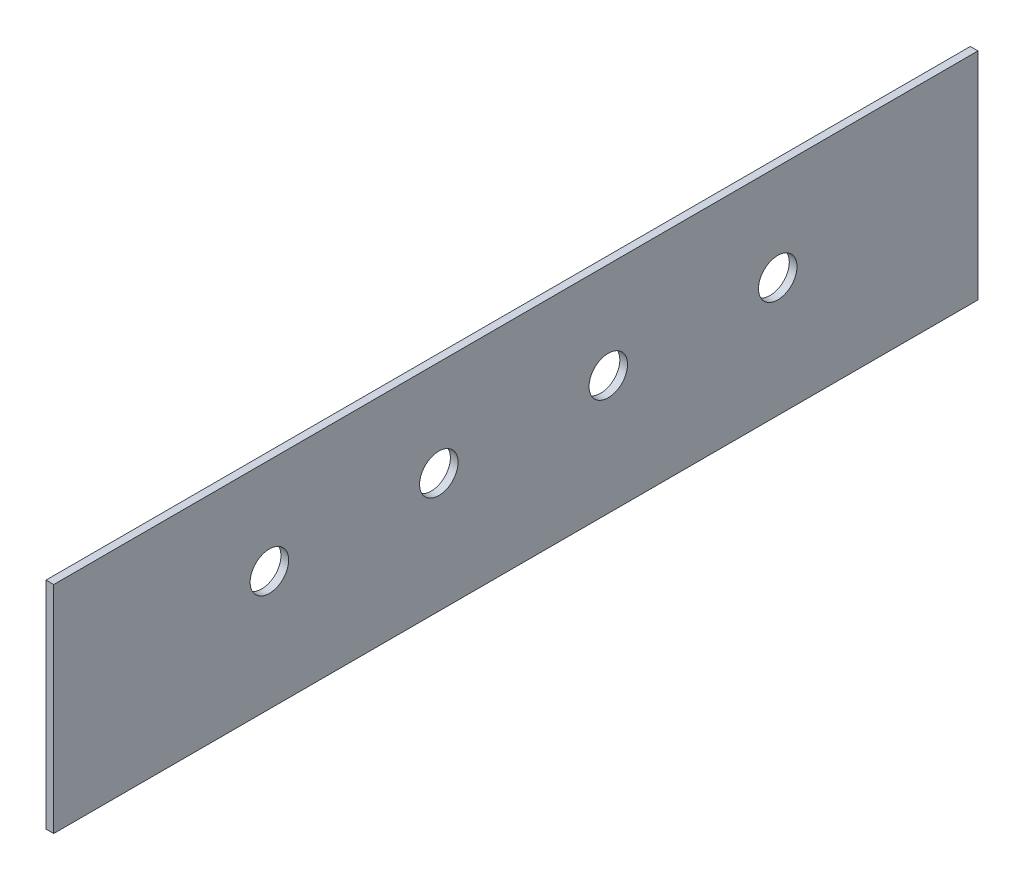
SolidWorks part; units mm, degrees
ref_plane "Front Plane" through (0, 0, 0) normal (0, 0, 1) x (1, 0, 0)
ref_plane "Top Plane" through (0, 0, 0) normal (0, 1, 0) x (1, 0, 0)
ref_plane "Right Plane" through (0, 0, 0) normal (1, 0, 0) x (0, 0, -1)
other "Configuration Table"
sketch "Sketch1" plane through (0, 0, 0) normal (1, 0, 0) x (0, 0, -1)
  line L1 (-600, -140) -> (600, -140)
  line L2 (-600, -140) -> (-600, 140)
  line L3 (-600, 140) -> (600, 140)
  line L4 (600, -140) -> (600, 140)
  line L5 (-600, -140) -> (600, 140) construction
  line L6 (-600, 140) -> (600, -140) construction
  point P0 (0, 0)
  dimension "D1" = 280
  dimension "D2" = 1200
extrude "Boss-Extrude1" add sketch "Sketch1" along normal blind 10
sketch "Sketch2" plane through (10, 0, 0) normal (1, 0, 0) x (0, 0, -1)
  line L0 (-600, 140) -> (-600, -140) construction
  line L1 (600, 140) -> (-600, 140) construction
  circle A0 centre (-320, 15) radius 25
  dimension "D1" = 50
  dimension "D2" = 280
  dimension "D3" = 125
extrude "Cut-Extrude1" cut sketch "Sketch2" against normal blind 10
pattern_linear "LPattern1" count 4 spacing 220 along (0, 0, -1) of "Cut-Extrude1"
